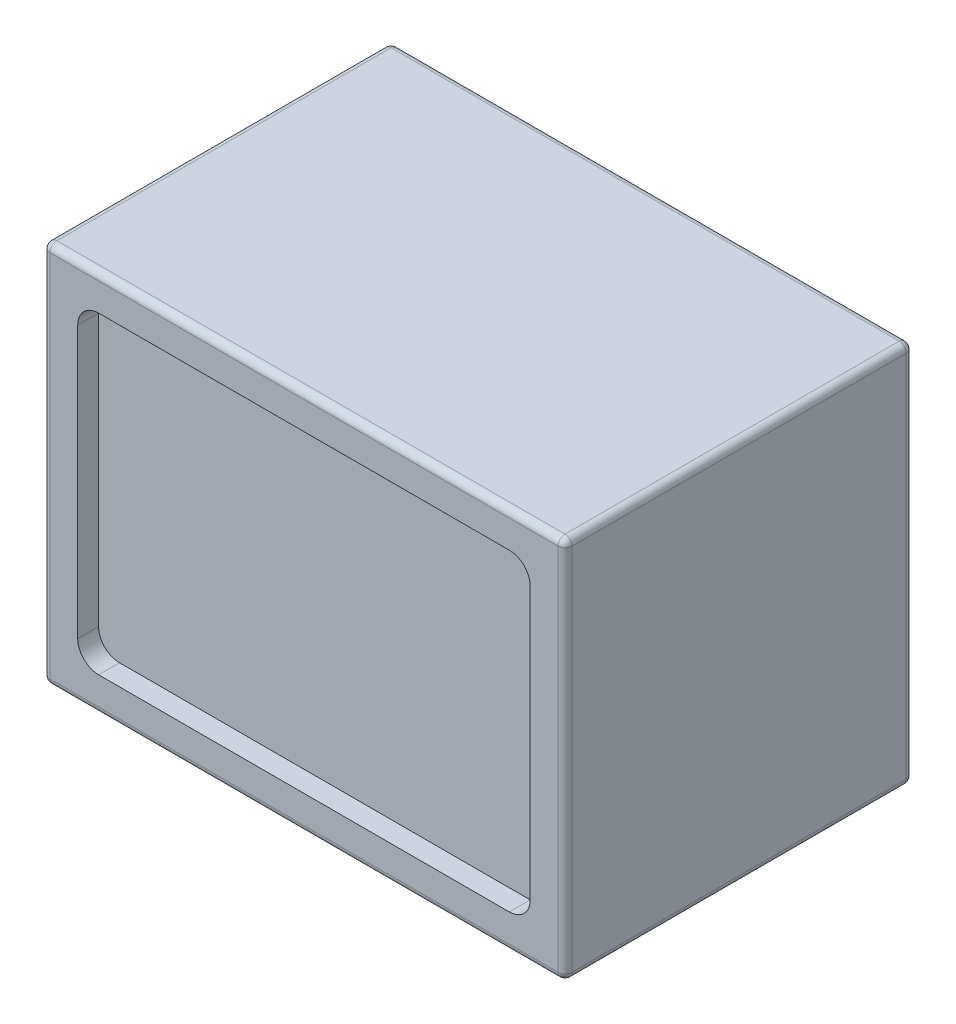
from build123d import *

# Parameters (mm, degrees)
SKETCH_1_W          = 75
SKETCH_1_H          = 55
EXTRUDE_1_DEPTH     = 50
SKETCH_2_W          = 65
SKETCH_2_H          = 45
CUT_EXTRUDE_1_DEPTH = 3
FILLET_1_R          = 3
FILLET_2_R          = 1


with BuildPart() as part:
    # 草图1 → 凸台-拉伸1 (new body)
    with BuildSketch(Plane.XY):
        with Locations((37.5, 27.5)):
            Rectangle(SKETCH_1_W, SKETCH_1_H)
    extrude(amount=EXTRUDE_1_DEPTH)

    # 草图2 → 切除-拉伸1 (cut)
    with BuildSketch(Plane.XY.offset(50)):
        with Locations((37.5, 27.5)):
            Rectangle(SKETCH_2_W, SKETCH_2_H)
    extrude(amount=-CUT_EXTRUDE_1_DEPTH, mode=Mode.SUBTRACT)

    # 圆角1
    fillet_1_edges = [part.edges().sort_by_distance(p)[0] for p in [
        (5, 5, 48.5),
        (5, 50, 48.5),
        (70, 50, 48.5),
        (70, 5, 48.5),
    ]]
    fillet(fillet_1_edges, radius=FILLET_1_R)

    # 圆角2
    fillet_2_edges = [part.edges().sort_by_distance(p)[0] for p in [
        (75, 27.5, 50),
        (37.5, 55, 50),
        (0, 27.5, 50),
        (37.5, 55, 0),
        (75, 27.5, 0),
        (37.5, 0, 0),
        (0, 27.5, 0),
        (0, 55, 25),
        (75, 55, 25),
        (75, 0, 25),
        (0, 0, 25),
        (37.5, 0, 50),
    ]]
    fillet(fillet_2_edges, radius=FILLET_2_R)


solid = part.part
